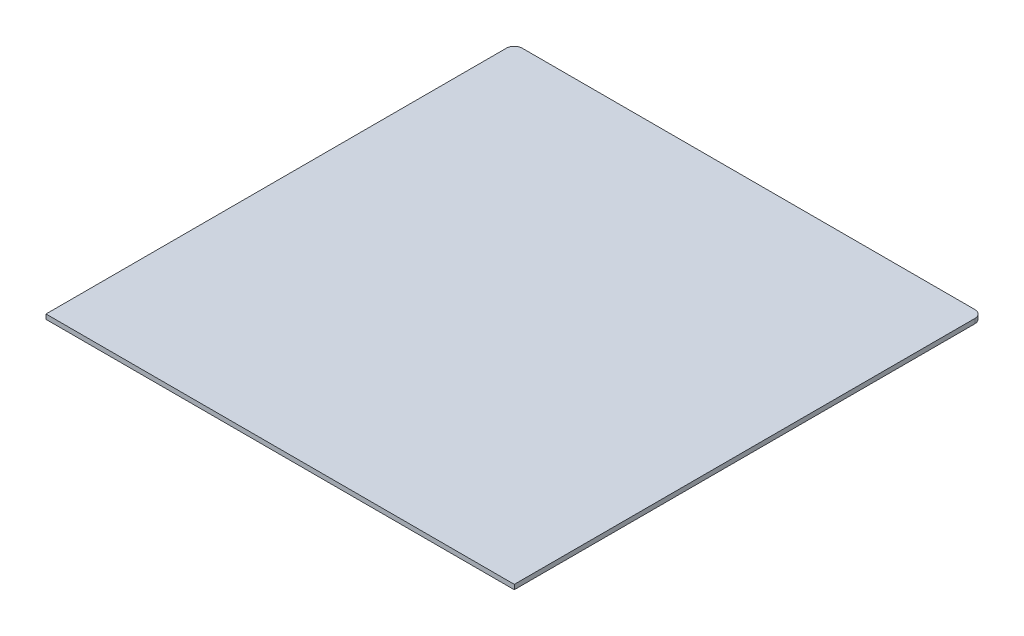
from build123d import *

# Parameters (mm, degrees)
BOSS_EXTRUDE1_DEPTH = 3


with BuildPart() as part:
    # Sketch1 → Boss-Extrude1 (new body)
    with BuildSketch(Plane(origin=(0, 0, 0), x_dir=(1, 0, 0), z_dir=(0, 1, 0))):
        with BuildLine():
            Line((-150, -150), (150, -150))
            Line((150, -150), (150, 145))
            ThreePointArc((150, 145), (148.535533906, 148.535533906), (145, 150))
            Line((145, 150), (-145, 150))
            ThreePointArc((-145, 150), (-148.535533906, 148.535533906), (-150, 145))
            Line((-150, 145), (-150, -150))
        make_face()
    extrude(amount=BOSS_EXTRUDE1_DEPTH)


solid = part.part
